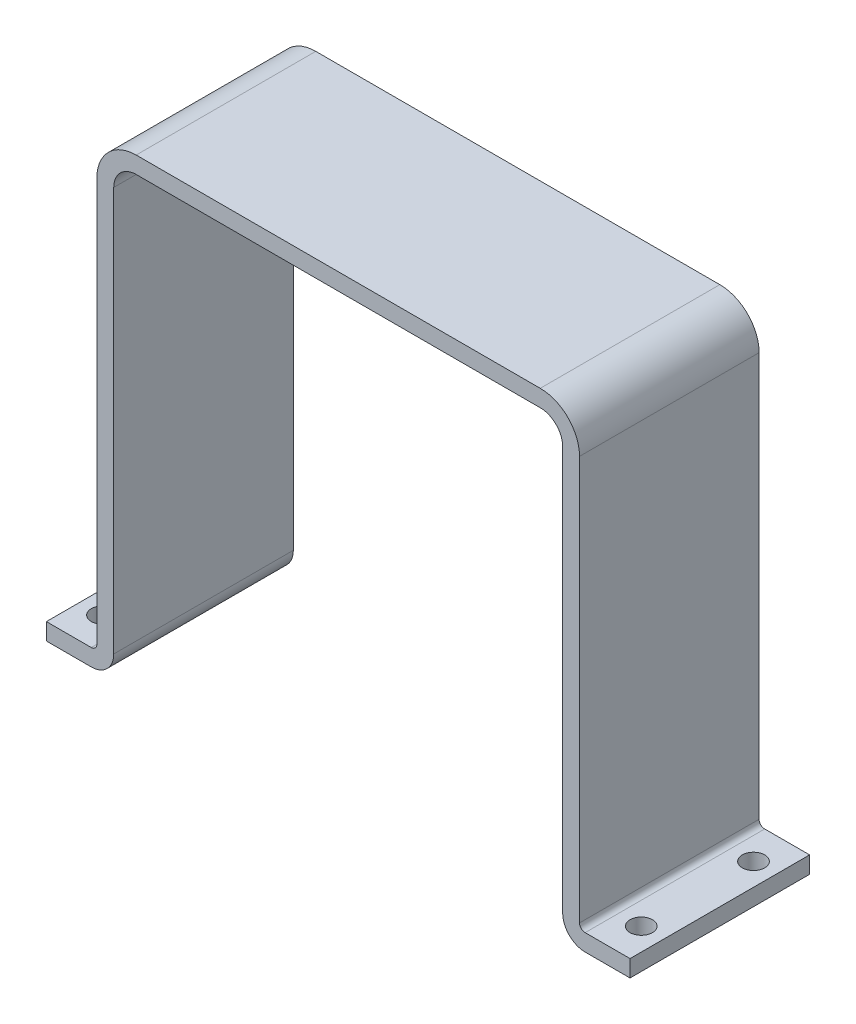
SolidWorks part; units mm, degrees
ref_plane "Front Plane" through (0, 0, 0) normal (0, 0, 1) x (1, 0, 0)
ref_plane "Top Plane" through (0, 0, 0) normal (0, 1, 0) x (1, 0, 0)
ref_plane "Right Plane" through (0, 0, 0) normal (1, 0, 0) x (0, 0, -1)
sketch "Sketch1" plane through (0, 0, 0) normal (0, 0, 1) x (1, 0, 0)
  line L0 (0, 0) -> (4, 0)
  line L1 (6, 2) -> (6, 38)
  line L2 (8, 40) -> (44, 40)
  line L3 (46, 38) -> (46, 2)
  line L4 (48, 0) -> (52, 0)
  line L5 (0, 1.5) -> (4, 1.5)
  line L6 (4.5, 2) -> (4.5, 38)
  line L7 (8, 41.5) -> (44, 41.5)
  line L8 (47.5, 38) -> (47.5, 2)
  line L9 (48, 1.5) -> (52, 1.5)
  line L10 (0, 1.5) -> (0, 0)
  line L11 (52, 1.5) -> (52, 0)
  arc A0 (46, 2) -> (48, 0) centre (48, 2) ccw
  arc A1 (6, 38) -> (8, 40) centre (8, 38) cw
  arc A2 (44, 40) -> (46, 38) centre (44, 38) cw
  arc A3 (4, 0) -> (6, 2) centre (4, 2) ccw
  arc A4 (4, 1.5) -> (4.5, 2) centre (4, 2) ccw
  arc A5 (4.5, 38) -> (8, 41.5) centre (8, 38) cw
  arc A6 (44, 41.5) -> (47.5, 38) centre (44, 38) cw
  arc A7 (47.5, 2) -> (48, 1.5) centre (48, 2) ccw
  point P9 (46, 0)
  point P12 (6, 40)
  point P15 (46, 40)
  point P18 (6, 0)
  dimension "D5" = 2
  dimension "D1" = 40
  dimension "D2" = 40
  dimension "D3" = 6
  dimension "D4" = 6
  dimension "D6" = 1.5
extrude "Boss-Extrude1" add sketch "Sketch1" along normal blind 16
sketch "Sketch2" plane through (0, 1.5, 0) normal (0, 1, 0) x (1, 0, 0)
  line L0 (52, -16) -> (52, 0) construction
  line L1 (52, 0) -> (48, 0) construction
  line L2 (52, -16) -> (48, -16) construction
  line L3 (4, -16) -> (0, -16) construction
  line L4 (0, -16) -> (0, 0) construction
  line L5 (4, 0) -> (0, 0) construction
  circle A0 centre (50, -3) radius 1
  circle A1 centre (50, -13) radius 1
  circle A2 centre (2, -3) radius 1
  circle A3 centre (2, -13) radius 1
  dimension "D1" = 2
  dimension "D2" = 2
  dimension "D3" = 2
  dimension "D4" = 2
  dimension "D5" = 2
  dimension "D6" = 3
  dimension "D7" = 2
  dimension "D8" = 3
  dimension "D9" = 3
  dimension "D10" = 2
  dimension "D12" = 3
  dimension "D11" = 2
extrude "Cut-Extrude1" cut sketch "Sketch2" against normal blind 16
